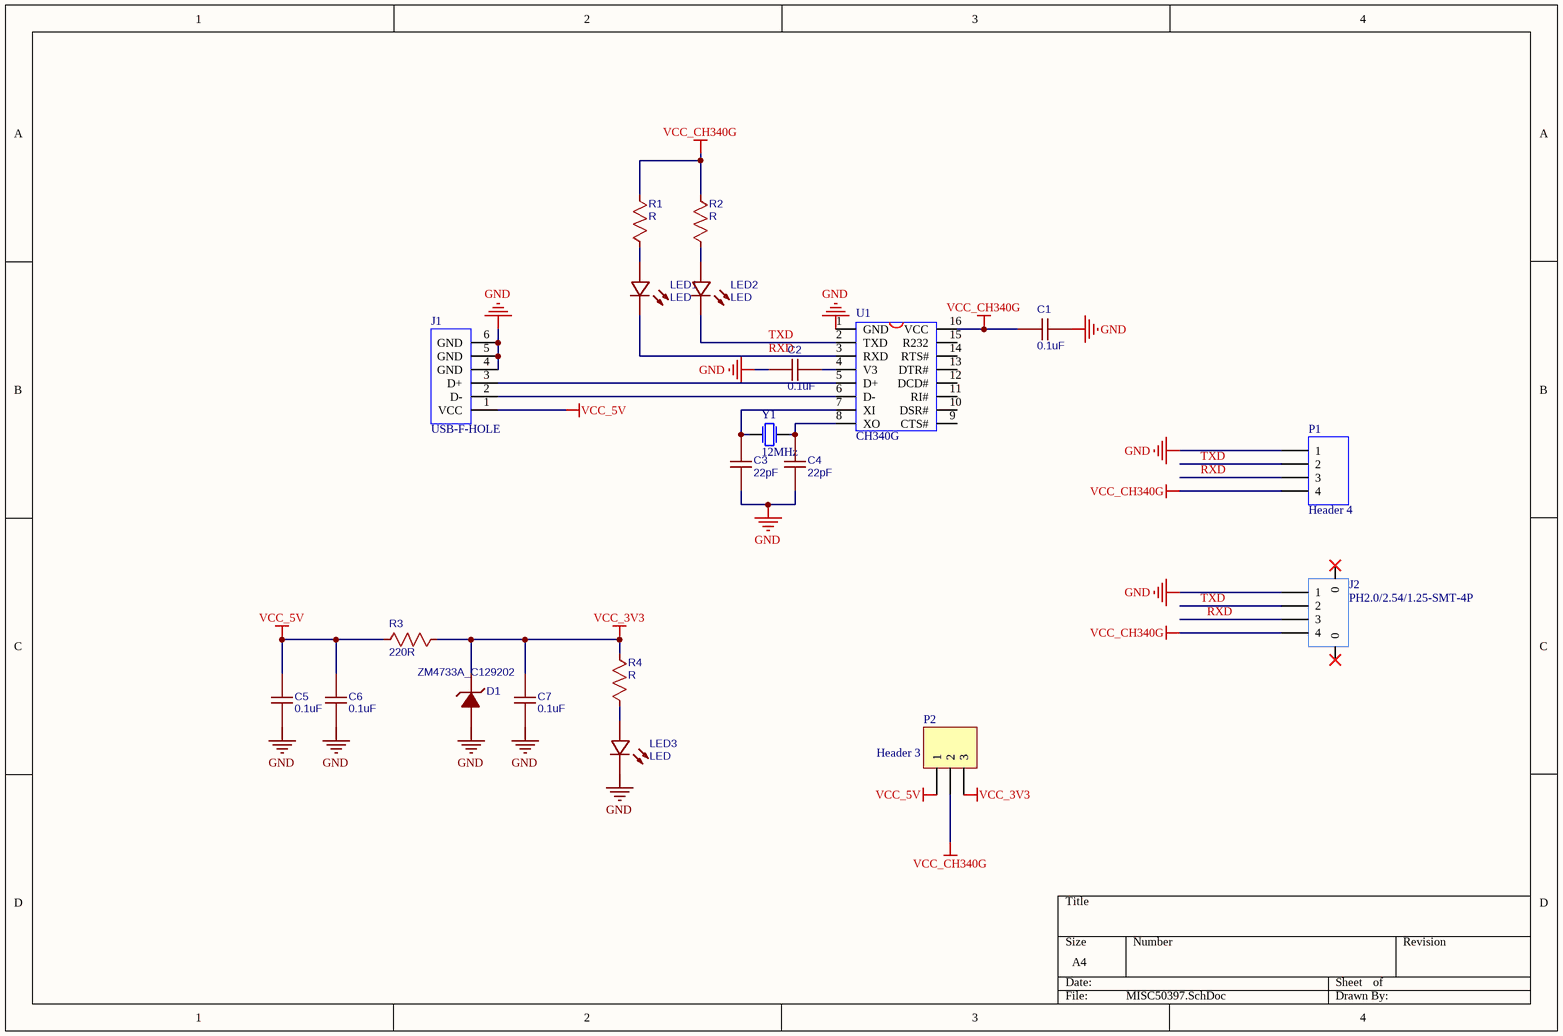
[diagram p0: MISC50397.SchDoc]
# Altium project MISC50397.PrjPCB
1 sheet, 21 parts. Net scope: global (net labels, ports and power ports of the same name join across sheets).
Board files: MISC50397-29.PcbDoc, MISC50397.PcbDoc

## Sheet MISC50397.SchDoc
size A4

### Parts
C1  0.1uF  [CAP0603]
C2  0.1uF  [CAP0603]
C3  22pF  [CAP0603]
C4  22pF  [CAP0603]
C5  0.1uF  [CAP0603]
C6  0.1uF  [CAP0603]
C7  0.1uF  [CAP0603]
D1  ZM4733A_C129202  [LL-41]
J1  USB-F-HOLE  [USB-F-HOLE]
J2  PH2.0/2.54/1.25-SMT-4P  [PH2.0-4P-WT]
LED1  LED  [LED-0603_RED]
LED2  LED  [LED-0603_RED]
LED3  LED  [LED-0603_RED]
P1  Header 4  [HDR1X4]
P2  Header 3  [HDR1X3]
R1  R  [RES0603]
R2  R  [RES0603]
R3  220R  [RES0603]
R4  R  [RES0603]
U1  CH340G  [SOP16M]
Y1  12MHz  [XTAL-5.08]

### Nets
GND: C1.2 C2.2 C3.1 C4.1 C5.1 C6.1 C7.1 D1.1(A) J1.4(GND) J1.5(GND) J1.6(GND) J2.1 LED3.2(-) P1.1 U1.1(GND)
VCC_3V3: C7.2 D1.2(K) P2.3 R3.2 R4.2
VCC_5V: C5.2 C6.2 J1.1(VCC) P2.1 R3.1
VCC_CH340G: C1.1 J2.4 P1.4 P2.2 R1.2 R2.2 U1.16(VCC)
RXD: J2.3 LED1.2(-) P1.3 U1.3(RXD)
TXD: J2.2 LED2.2(-) P1.2 U1.2(TXD)
NetC2_1: C2.1 U1.4(V3)
NetC3_2: C3.2 U1.7(XI) Y1.2(P2)
NetC4_2: C4.2 U1.8(XO) Y1.1(P1)
NetJ1_2: J1.2(D-) U1.6(D-)
NetJ1_3: J1.3(D+) U1.5(D+)
NetLED1_1: LED1.1(+) R1.1
NetLED2_1: LED2.1(+) R2.1
NetLED3_1: LED3.1(+) R4.1

Not connected (* = marked no-connect by the designer): J2 0*; U1 9(CTS#) 10(DSR#) 11(RI#) 12(DCD#) 13(DTR#) 14(RTS#) 15(R232)

### Library data of the parts
C1-C7 = C: BOM_Manufacturer: SEIKO; BOM_Manufacturer Part: XH414HG-IV01E; nameAlias: Capacitance; BOM_Supplier: LCSC; BOM_Supplier Part: C38065; spicePre: C; spiceSymbolName: XH414HG-IV01E
D1 = ZM4733A_C129202: BOM_Manufacturer: Tak Cheong; Contributor: LCSC; BOM_Supplier: LCSC; BOM_Supplier Part: C129202; BOM_Manufacturer Part: ZM4733A; spicePre: D
LED1-LED3 = LED: BOM_Manufacturer: EVERLIGHT; BOM_Manufacturer Part: 204-10SURD/S530-A3; BOM_Supplier: LCSC; BOM_Supplier Part: C99772; spicePre: L
P1 = Header 4: Header, 4-Pin; LatestRevisionDate: 17-Jul-2002; LatestRevisionNote: Re-released for DXP Platform.; Publisher: Altium Limited
P2 = Header 3: Header, 3-Pin; LatestRevisionDate: 17-Jul-2002; LatestRevisionNote: Re-released for DXP Platform.; Publisher: Altium Limited
R1-R4 = R: nameAlias: Value(Ω); BOM_Manufacturer Part: ?; spicePre: R; spiceSymbolName: Res_AXIAL-0.3(1/8W)_US
U1 = CH340G: USB2UART
Y1 = XTAL